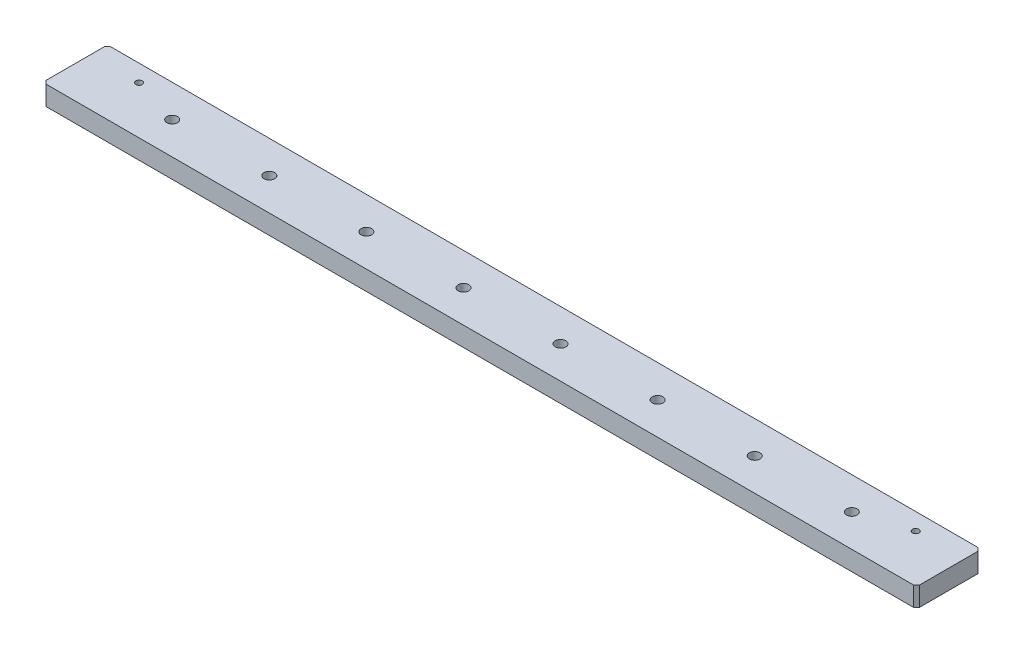
from build123d import *

# Parameters (mm, degrees)
SKETCH_1_W                   = 540
SKETCH_1_H                   = 40
EXTRUDE_1_DEPTH              = 12
CHAMFER_1_SIZE               = 2
F_4_0MM_1_D                  = 4
F_4_0MM_1_DEPTH              = 12
F_4_0MM_1_TIP                = 1.201721238
PATTERN_LINEAR_4_COUNT       = 9
PATTERN_LINEAR_4_PITCH       = 60
HOLE_WIZARD_M6_1_D           = 6.6
HOLE_WIZARD_M6_1_CBORE_D     = 11
HOLE_WIZARD_M6_1_CBORE_DEPTH = 6.8
PATTERN_LINEAR_5_COUNT       = 8
PATTERN_LINEAR_5_PITCH       = 60


with BuildPart() as part:
    # 草图1 → 凸台-拉伸1 (new body)
    with BuildSketch(Plane(origin=(0, 0, 0), x_dir=(1, 0, 0), z_dir=(0, 1, 0))):
        Rectangle(SKETCH_1_W, SKETCH_1_H)
    extrude(amount=EXTRUDE_1_DEPTH)

    # 倒角1
    chamfer_1_edges = [part.edges().sort_by_distance(p)[0] for p in [
        (270, 6, 20),
        (-270, 6, 20),
        (-270, 6, -20),
        (270, 6, -20),
    ]]
    chamfer(chamfer_1_edges, length=CHAMFER_1_SIZE)

    # Ø4.0mm 暗销孔1
    with Locations(Plane(origin=(0, 0, 0), x_dir=(-1, 0, 0), z_dir=(0, -1, 0))):
        with Locations((-240, 9.5), (240, 9.5)):
            Hole(F_4_0MM_1_D / 2, depth=F_4_0MM_1_DEPTH)
            with Locations((0, 0, -(F_4_0MM_1_DEPTH + F_4_0MM_1_TIP / 2))):  # 118° drill point
                Cone(0, F_4_0MM_1_D / 2, F_4_0MM_1_TIP, mode=Mode.SUBTRACT)

    # 草图6 → M3 螺纹孔1 (revolve, cut)
    with BuildSketch(Plane(origin=(240, 0, 0), x_dir=(0, 0, -1), z_dir=(1, 0, 0))):
        Polygon((0, 0), (0, 8.251075774), (1.25, 7.5), (1.25, 0), align=None)
    hole_wizard_m3_1 = revolve(axis=Axis((240, -6.35, 0), (0, 1, 0)), mode=Mode.SUBTRACT)

    # 阵列(线性)4: M3 螺纹孔1 ×9
    with Locations(*[(-i * PATTERN_LINEAR_4_PITCH, 0, 0) for i in range(1, PATTERN_LINEAR_4_COUNT)]):
        add(hole_wizard_m3_1, mode=Mode.SUBTRACT)

    # M6 六角圆柱头螺钉的柱形沉头孔1 (through all)
    with Locations(Plane(origin=(0, 0, 0), x_dir=(-1, 0, 0), z_dir=(0, -1, 0))):
        with Locations((210, 0)):
            hole_wizard_m6_1 = CounterBoreHole(HOLE_WIZARD_M6_1_D / 2, HOLE_WIZARD_M6_1_CBORE_D / 2, HOLE_WIZARD_M6_1_CBORE_DEPTH)

    # 阵列(线性)5: M6 六角圆柱头螺钉的柱形沉头孔1 ×8
    with Locations(*[(i * PATTERN_LINEAR_5_PITCH, 0, 0) for i in range(1, PATTERN_LINEAR_5_COUNT)]):
        add(hole_wizard_m6_1, mode=Mode.SUBTRACT)


solid = part.part
